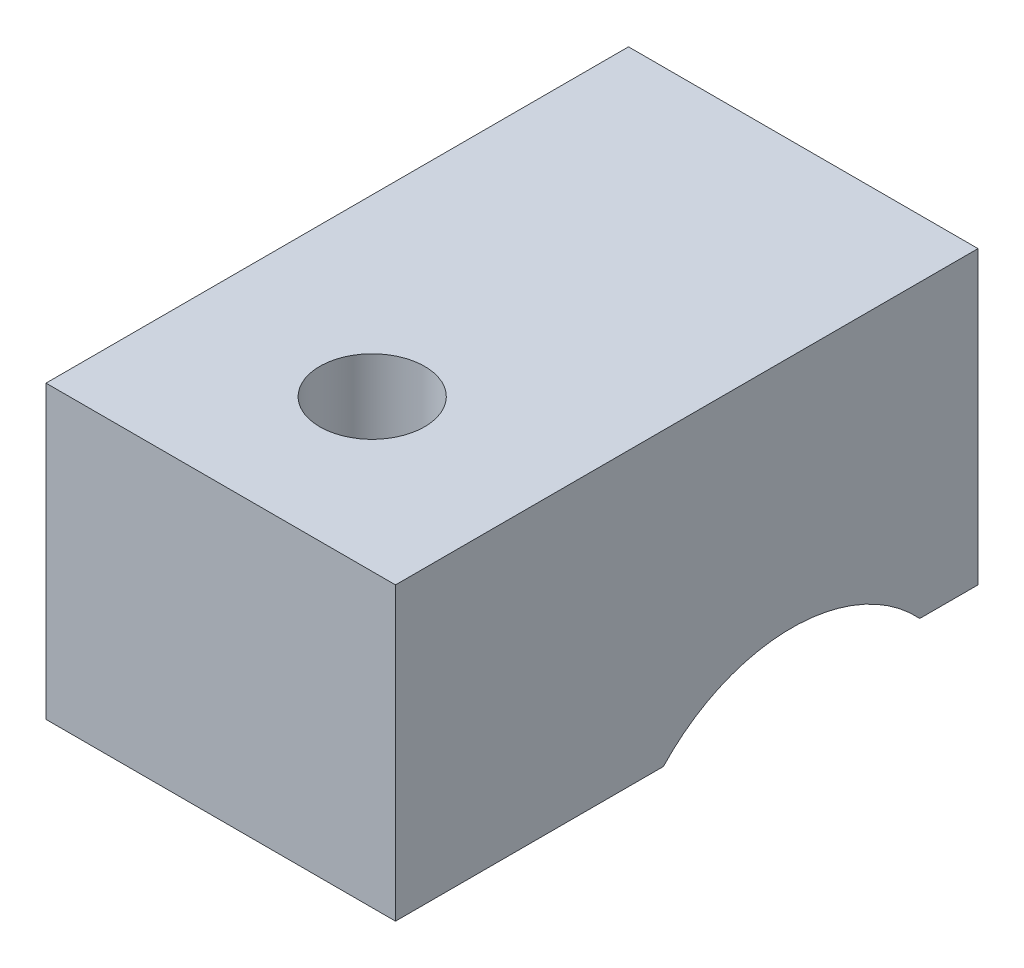
from build123d import *

# Parameters (mm, degrees)
SKETCH1_W              = 30
SKETCH1_H              = 25
BOSS_EXTRUDE1_DEPTH    = 50
CUT_EXTRUDE1_DEPTH     = 95
M10X1_0_TAPPED_HOLE1_D = 9


with BuildPart() as part:
    # Sketch1 → Boss-Extrude1 (new body)
    with BuildSketch(Plane.XY):
        with Locations((15, 12.5)):
            Rectangle(SKETCH1_W, SKETCH1_H)
    extrude(amount=BOSS_EXTRUDE1_DEPTH)

    # Sketch2 → Cut-Extrude1 (cut)
    with BuildSketch(Plane(origin=(30, 30, 0), x_dir=(0, -1, 0), z_dir=(-1, 0, 0))):
        with BuildLine():
            Line((30, 27), (30, 5))
            ThreePointArc((30, 5), (25.198039027, 16), (30, 27))
        make_face()
    extrude(amount=CUT_EXTRUDE1_DEPTH, mode=Mode.SUBTRACT)

    # M10x1.0 Tapped Hole1 (through all)
    with Locations(Plane(origin=(0, 25, 0), x_dir=(-1, 0, 0), z_dir=(0, 1, 0))):
        with Locations((-15, 37)):
            Hole(M10X1_0_TAPPED_HOLE1_D / 2)


solid = part.part
